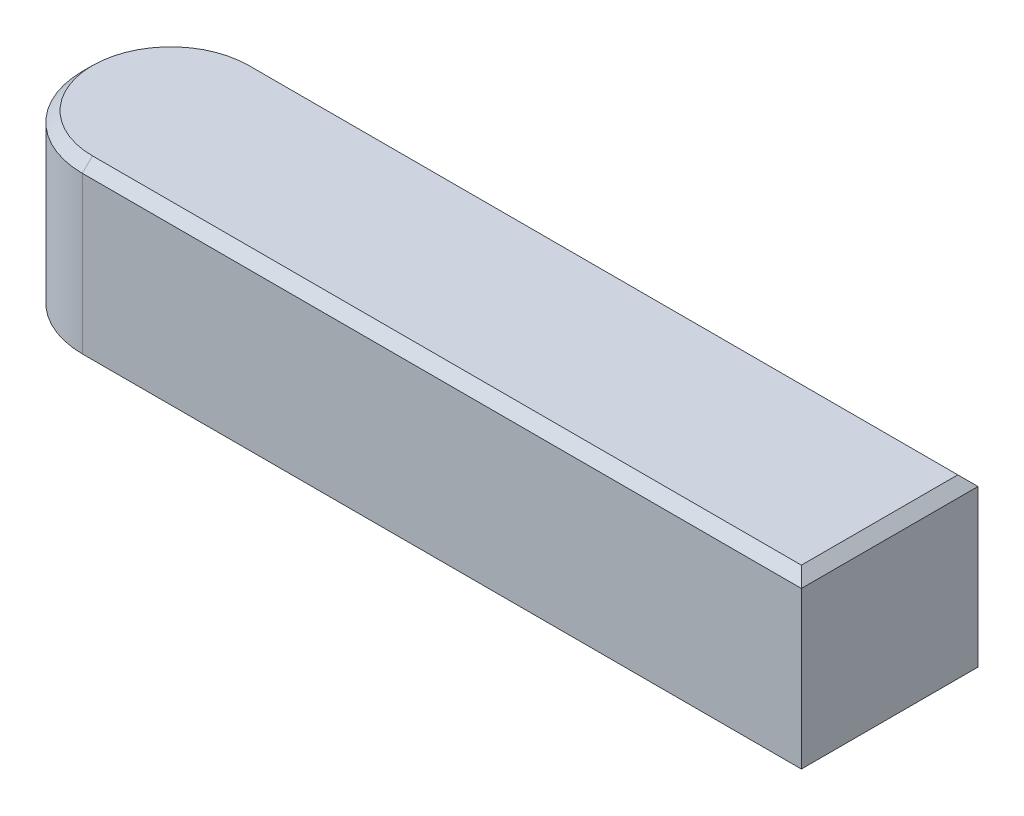
SolidWorks part; units mm, degrees
ref_plane "前视基准面" through (0, 0, 0) normal (0, 0, 1) x (1, 0, 0)
ref_plane "上视基准面" through (0, 0, 0) normal (0, 1, 0) x (1, 0, 0)
ref_plane "右视基准面" through (0, 0, 0) normal (1, 0, 0) x (0, 0, -1)
sketch "草图1" plane through (0, 0, 0) normal (0, 1, 0) x (1, 0, 0)
  line L1 (3.5, 0) -> (32, 0)
  line L3 (3.5, -7) -> (32, -7)
  line L4 (32, 0) -> (32, -7)
  arc A0 (3.5, 0) -> (3.5, -7) centre (3.5, -3.5) ccw
  dimension "D3" = 7
  dimension "D1" = 28.5
extrude "凸台-拉伸1" add sketch "草图1" along normal blind 7 contours L3 L4 L1 A0
chamfer "倒角1" distance 0.4 angle 45 8 edges at (32, 7, 3.5) (17.75, 7, 7) (17.75, 7, 0) (0, 7, 3.5) (32, 0, 3.5) (17.75, 0, 0) (17.75, 0, 7) (0, 0, 3.5)
